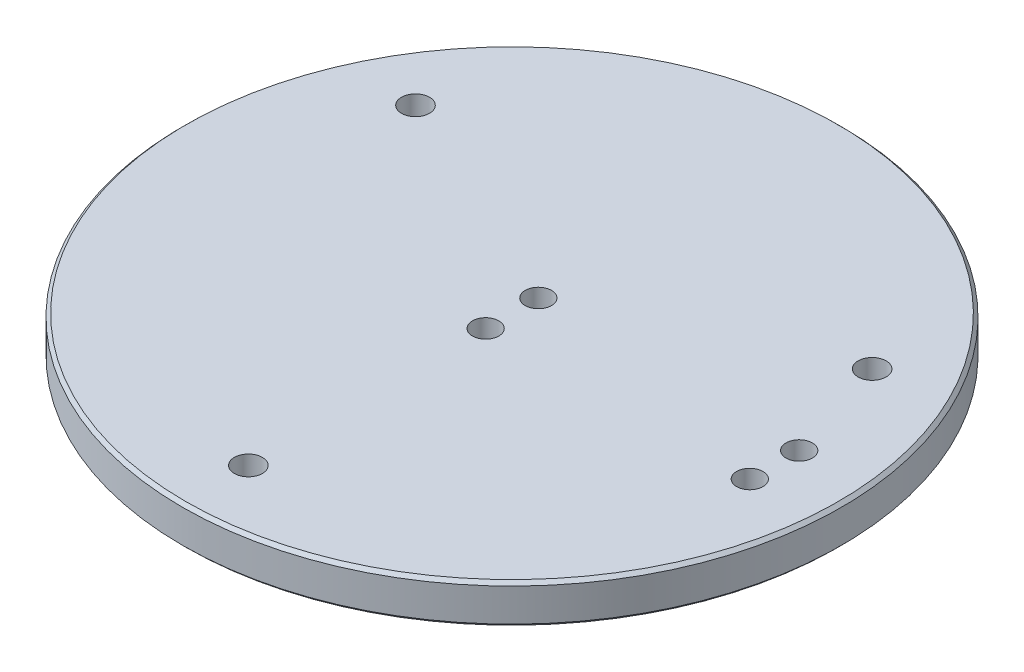
SolidWorks part; units mm, degrees
material "Q235"
ref_plane "Front Plane" through (0, 0, 0) normal (0, 0, 1) x (1, 0, 0)
ref_plane "Top Plane" through (0, 0, 0) normal (0, 1, 0) x (1, 0, 0)
ref_plane "Right Plane" through (0, 0, 0) normal (1, 0, 0) x (0, 0, -1)
sketch "Sketch2" plane through (0, 0, 0) normal (0, 1, 0) x (1, 0, 0)
  line L0 (-69.282, 40) -> (0, 0) construction
  line L1 (0, 0) -> (0, -80) construction
  line L2 (0, 0) -> (-119.531, 0) construction
  circle A0 centre (0, 0) radius 100
  circle A1 centre (0, 0) radius 80 construction
  point P5 (0, 8)
  point P6 (0, -80)
  point P8 (-69.282, 40)
  point P9 (69.282, 40)
  point P10 (0, 0)
  point P11 (0, -8)
  point P12 (79.6477, 7.5)
  point P13 (79.6477, -7.5)
  dimension "D1" = 200
  dimension "D2" = 160
  dimension "D4" = 120
  dimension "D5" = 15
  dimension "D6" = 16
  dimension "D7" = 8
  dimension "D8" = 7.5
  dimension "D3" = 3
extrude "Boss-Extrude1" add sketch "Sketch2" against normal blind 12 contours A0
hole_wizard "M10 Tapped Hole1" positions "3DSketch2" profile "Sketch3" tap size "M10" standard "GB"
sketch3d "3DSketch2"
  point P0 (-69.282, 0, -40)
  point P2 (69.282, 0, -40)
  point P4 (0, 0, 80)
sketch "Sketch3" plane through (-69.282, 0, -40) normal (1, 0, 0) x (0, 0, 1)
  line L0 (0, 0) -> (0, 27.0537)
  line L1 (0, 27.0537) -> (4.25, 24.5)
  line L2 (4.25, 24.5) -> (4.25, 0)
  line L5 (4.25, 0) -> (0, 0)
  line L10 (0, 27.0537) -> (-4.25, 24.5) construction
  line L11 (0, -6.35) -> (0, 107.95) construction
  dimension "螺纹孔钻头直径" = 8.5
  dimension "螺纹孔钻头深度" = 24.5
  dimension "导头角度" = 118
cosmetic thread "Cosmetic Thread3"
cosmetic thread "Cosmetic Thread4"
cosmetic thread "Cosmetic Thread5"
hole_wizard "CBORE for M4 Hex Head Bolt1" positions "3DSketch3" profile "Sketch4" counterbore size "M4" standard "GB"
sketch3d "3DSketch3"
  point P3 (79.6477, 0, -7.5)
  point P5 (79.6477, 0, 7.5)
  point P7 (0, 0, 8)
  point P9 (0, 0, -8)
sketch "Sketch4" plane through (79.6477, 0, -7.5) normal (1, 0, 0) x (0, 0, 1)
  line L0 (0, 0) -> (0, 25.8519)
  line L1 (0, 25.8519) -> (2.25, 24.5)
  line L2 (2.25, 24.5) -> (2.25, 7)
  line L3 (2.25, 7) -> (4, 7)
  line L4 (4, 7) -> (4, 0)
  line L5 (4, 0) -> (0, 0)
  line L10 (0, 25.8519) -> (-2.25, 24.5) construction
  line L11 (0, -6.35) -> (0, 107.95) construction
  dimension "孔直径" = 4.5
  dimension "孔深度" = 24.5
  dimension "柱形沉头孔直径" = 8
  dimension "柱形沉头孔深度" = 7
  dimension "导头角度" = 118
chamfer "Chamfer1" distance 1 angle 45 2 edges at (0, 0, 100) (0, -12, 100)
